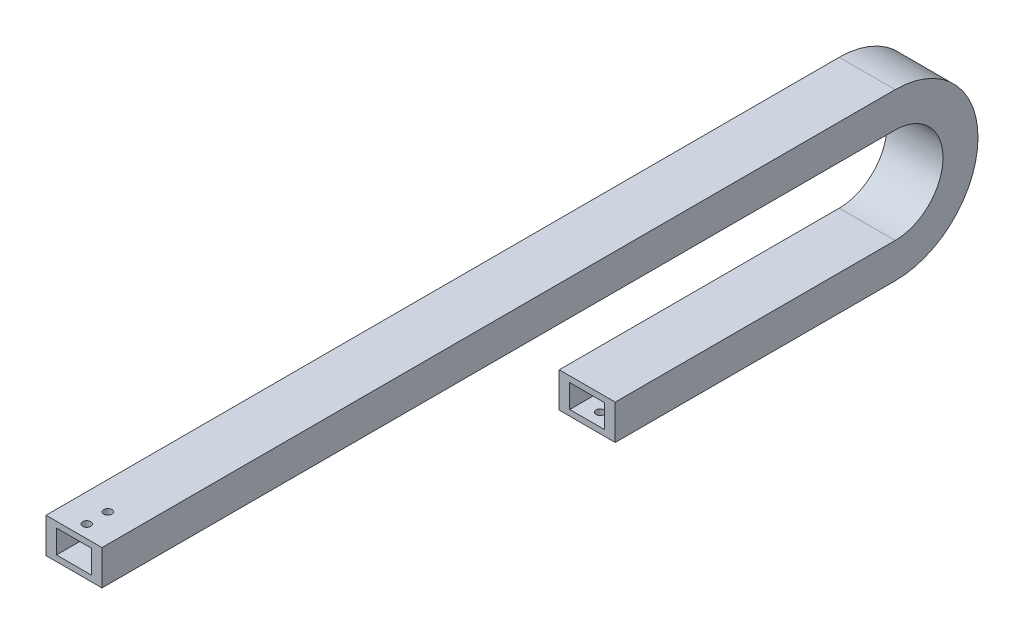
SolidWorks part; units mm, degrees
ref_plane "前视基准面" through (0, 0, 0) normal (0, 0, 1) x (1, 0, 0)
ref_plane "上视基准面" through (0, 0, 0) normal (0, 1, 0) x (1, 0, 0)
ref_plane "右视基准面" through (0, 0, 0) normal (1, 0, 0) x (0, 0, -1)
sketch "草图1" plane through (0, 0, 0) normal (0, 0, 1) x (1, 0, 0)
  line L1 (12, -7.5) -> (-12, -7.5)
  line L2 (12, -7.5) -> (12, 7.5)
  line L3 (12, 7.5) -> (-12, 7.5)
  line L4 (-12, -7.5) -> (-12, 7.5)
  line L5 (12, -7.5) -> (-12, 7.5) construction
  line L6 (12, 7.5) -> (-12, -7.5) construction
  line L7 (7.5, -5) -> (-7.5, -5)
  line L8 (7.5, -5) -> (7.5, 5)
  line L9 (7.5, 5) -> (-7.5, 5)
  line L10 (-7.5, -5) -> (-7.5, 5)
  line L11 (7.5, -5) -> (-7.5, 5) construction
  line L12 (7.5, 5) -> (-7.5, -5) construction
  point P0 (0, 0)
  point P6 (0, 0)
  dimension "D1" = 24
  dimension "D2" = 15
  dimension "D3" = 15
  dimension "D4" = 10
sketch "草图2" plane through (0, 0, 0) normal (1, 0, 0) x (0, 0, -1)
  line L0 (0, 0) -> (120, 0)
  line L1 (120, 56) -> (-220, 56)
  arc A0 (120, 0) -> (120, 56) centre (120, 28) ccw
  dimension "D1" = 28
  dimension "D2" = 340
  dimension "D3" = 120
sweep "扫描1" add profiles "草图1" path "草图2"
sketch "草图3" plane through (0, 63.5, 0) normal (0, 1, 0) x (1, 0, 0)
  line L0 (-12, 120) -> (-12, -220) construction
  line L1 (-12, -220) -> (12, -220) construction
  circle A0 centre (0, -214.5) radius 1.75
  circle A1 centre (0, -205.5) radius 1.75
  dimension "D1" = 9
  dimension "D2" = 3.5
  dimension "D3" = 12
  dimension "D4" = 5.5
extrude "切除-拉伸1" cut sketch "草图3" against normal blind 5
sketch "草图4" plane through (0, -7.5, 0) normal (0, -1, 0) x (1, 0, 0)
  line L0 (-12, 0) -> (12, 0) construction
  line L1 (12, -120) -> (12, 0) construction
  circle A0 centre (0, -5.5) radius 1.75
  circle A1 centre (0, -14.5) radius 1.75
  dimension "D1" = 3.5
  dimension "D4" = 9
  dimension "D2" = 5.5
  dimension "D3" = 12
extrude "切除-拉伸2" cut sketch "草图4" against normal blind 5
